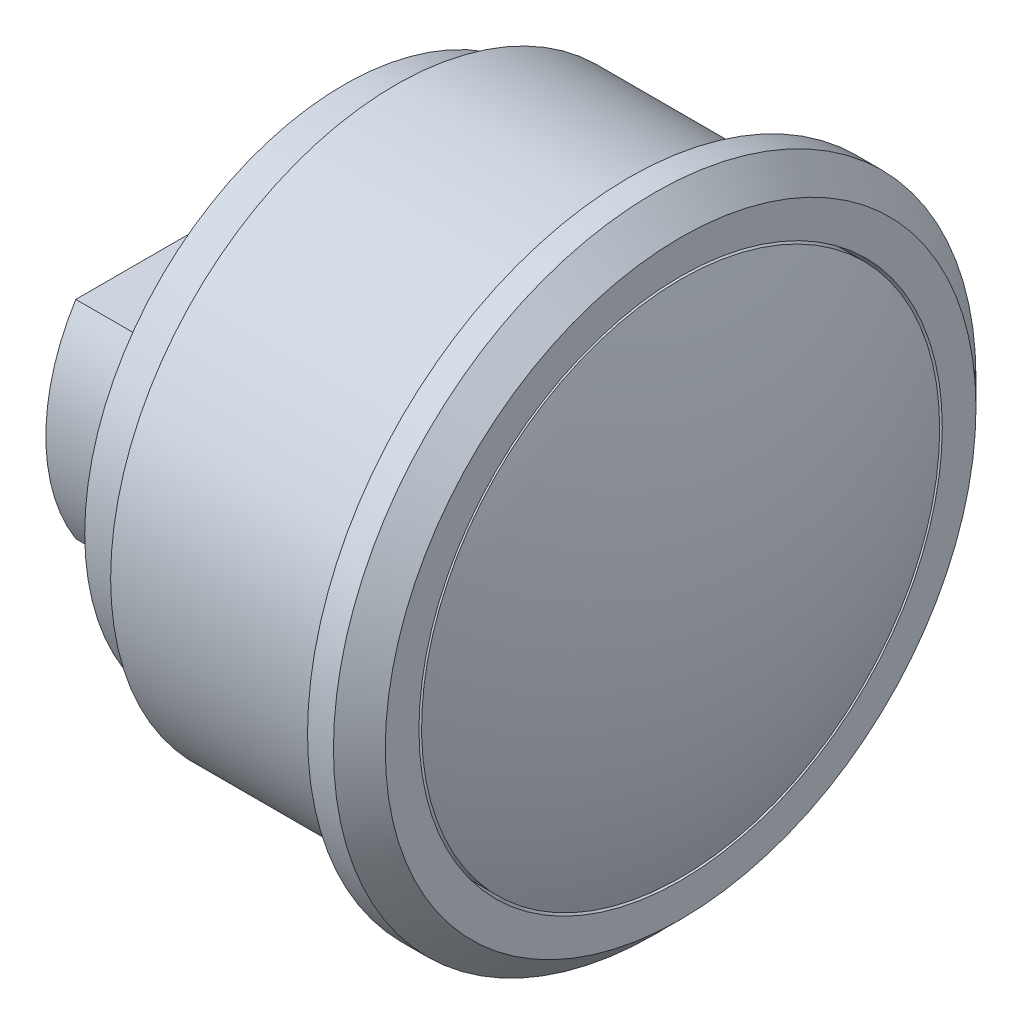
from build123d import *

# Parameters (mm, degrees)
CHAMFER1_SIZE       = 1
SKETCH5_OUTSIDE_W   = 34.778
SKETCH5_OUTSIDE_H   = 34.778
SKETCH5_OUTSIDE_W_2 = 16.801740482
SKETCH5_OUTSIDE_H_2 = 8
CUT_EXTRUDE2_DEPTH  = 4
CUT_EXTRUDE3_START  = -3
SKETCH7_R           = 10.1
SKETCH7_R_2         = 10
CUT_EXTRUDE3_DEPTH  = 3


with BuildPart() as part:
    # Sketch1 → Revolve1 (revolve)
    with BuildSketch(Plane(origin=(0, 0, 0), x_dir=(1, 0, 0), z_dir=(0, 1, 0)), mode=Mode.PRIVATE) as revolve1_sk:
        Polygon((0, 0), (17, 0), (17, 12.4), (15, 12.4), (15, 11), (6, 11), (6, 10), (4, 10), (4, 7.5), (0, 7.5), align=None)
    revolve(revolve1_sk.sketch.rotate(Axis((0, 0, 0), (1, 0, 0)), 180), axis=Axis((0, 0, 0), (1, 0, 0)))

    # Sketch3 → Revolve2 (revolve)
    with BuildSketch(Plane.XY):
        with BuildLine():
            Line((9, 0), (9, 10))
            Line((9, 10), (17, 10))
            ThreePointArc((17, 10), (18.495097568, 5.099019514), (19, 0))
            Line((19, 0), (9, 0))
        make_face()
    revolve(axis=Axis((9, 0, 0), (1, 0, 0)))

    # Chamfer1
    chamfer1_edges = [part.edges().sort_by_distance(p)[0] for p in [
        (17, 0, -12.4),
    ]]
    chamfer(chamfer1_edges, length=CHAMFER1_SIZE)

    # Sketch5 outside → Cut-Extrude2 (cut)
    with BuildSketch(Plane.ZY):
        Rectangle(SKETCH5_OUTSIDE_W, SKETCH5_OUTSIDE_H)
        Rectangle(SKETCH5_OUTSIDE_W_2, SKETCH5_OUTSIDE_H_2, mode=Mode.SUBTRACT)
    extrude(amount=-CUT_EXTRUDE2_DEPTH, mode=Mode.SUBTRACT)

    # Sketch7 → Cut-Extrude3 (cut)
    with BuildSketch(Plane(origin=(17, 0, 0), x_dir=(0, 0, -1), z_dir=(1, 0, 0)).offset(CUT_EXTRUDE3_START)):
        Circle(SKETCH7_R)
        with Locations(Location((0, 0, 0), (0, 0, 180))):
            Circle(SKETCH7_R_2, mode=Mode.SUBTRACT)
    extrude(amount=CUT_EXTRUDE3_DEPTH, mode=Mode.SUBTRACT)


solid = part.part
